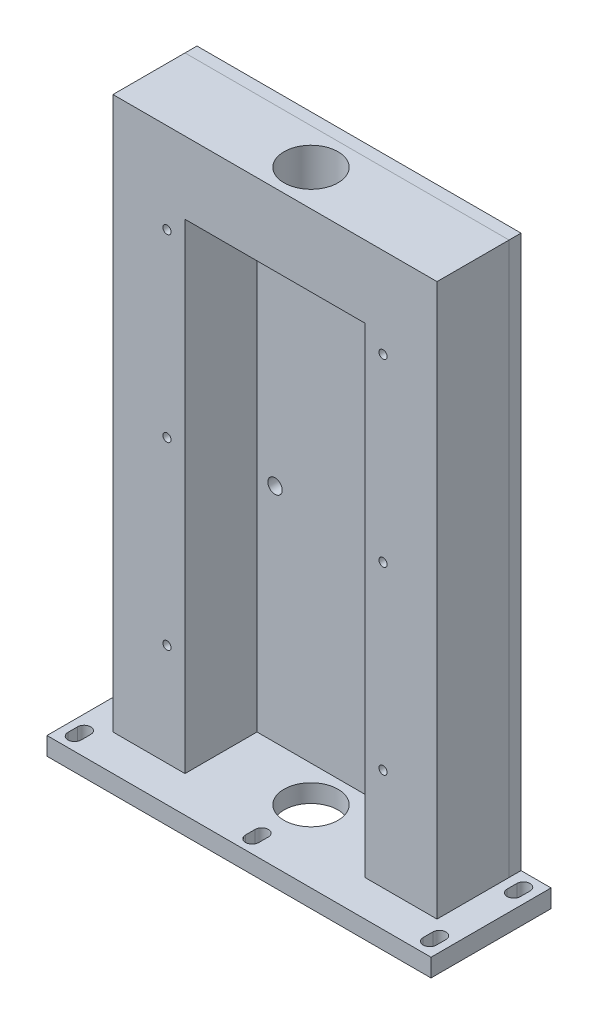
from build123d import *

# Parameters (mm, degrees)
BOSS_EXTRUDE1_DEPTH        = 60
SKETCH3_W                  = 270
SKETCH3_H                  = 460
BOSS_EXTRUDE3_DEPTH        = 10
SKETCH4_W                  = 320
SKETCH4_H                  = 100
BOSS_EXTRUDE4_DEPTH        = 15
SKETCH7_R                  = 5.5
CUT_EXTRUDE1_DEPTH         = 496.277699882
CUT_EXTRUDE3_DEPTH         = 496.277699882
SKETCH23_R                 = 22.5
CUT_EXTRUDE4_DEPTH         = 510.239629251
SKETCH24_R                 = 15
CUT_EXTRUDE5_DEPTH         = 498.192115786
SKETCH27_W                 = 3.4
SKETCH27_H                 = 100
M8_TAPPED_HOLE1_AT_2_COUNT = 2
M8_TAPPED_HOLE1_AT_2_PITCH = 180
M8_TAPPED_HOLE1_AT_3_COUNT = 2
M8_TAPPED_HOLE1_AT_3_PITCH = 150
M8_TAPPED_HOLE1_AT_4_COUNT = 2
M8_TAPPED_HOLE1_AT_4_PITCH = 234.307490277
M8_TAPPED_HOLE1_AT_5_COUNT = 2
M8_TAPPED_HOLE1_AT_5_PITCH = 300
M8_TAPPED_HOLE1_AT_6_COUNT = 2
M8_TAPPED_HOLE1_AT_6_PITCH = 349.857113691
SKETCH29_R                 = 6
CUT_EXTRUDE6_DEPTH         = 10


with BuildPart() as part:
    # Sketch1 → Boss-Extrude1 (new body)
    with BuildSketch(Plane.XY):
        Polygon((-135, 460), (135, 460), (135, 0), (75, 0), (75, 400), (-75, 400), (-75, 0), (-135, 0), align=None)
    extrude(amount=BOSS_EXTRUDE1_DEPTH)


with BuildPart() as body_2:
    # Sketch3 → Boss-Extrude3 (new body)
    with BuildSketch(Plane(origin=(0, 0, 0), x_dir=(-1, 0, 0), z_dir=(0, 0, -1))):
        with Locations((0, 230)):
            Rectangle(SKETCH3_W, SKETCH3_H)
    extrude(amount=BOSS_EXTRUDE3_DEPTH)

    # Sketch24 → Cut-Extrude5 (cut, through all)
    with BuildSketch(Plane(origin=(0, 0, -10), x_dir=(-1, 0, 0), z_dir=(0, 0, -1))):
        with Locations((-60, 257)):
            Circle(SKETCH24_R)
    extrude(amount=-CUT_EXTRUDE5_DEPTH, mode=Mode.SUBTRACT)


with BuildPart() as body_3:
    # Sketch4 → Boss-Extrude4 (new body)
    with BuildSketch(Plane.XZ):
        with Locations((0, 40)):
            Rectangle(SKETCH4_W, SKETCH4_H)
    extrude(amount=BOSS_EXTRUDE4_DEPTH)

    # Sketch7 → Cut-Extrude1 (cut, through all)
    with BuildSketch(Plane(origin=(0, 0, 0), x_dir=(1, 0, 0), z_dir=(0, 1, 0))):
        with Locations(Location((148, -5, 0), (0, 0, 270))):
            Circle(SKETCH7_R)
        with Locations(Location((148, -75, 0), (0, 0, 90))):
            Circle(SKETCH7_R)
        with Locations(Location((-148, -75, 0), (0, 0, 270))):
            Circle(SKETCH7_R)
        with Locations(Location((-148, -5, 0), (0, 0, 90))):
            Circle(SKETCH7_R)
        with Locations(Location((0, -75, 0), (0, 0, 270))):
            Circle(SKETCH7_R)
    extrude(amount=-CUT_EXTRUDE1_DEPTH, mode=Mode.SUBTRACT)

    # Sketch22 → Cut-Extrude3 (cut, through all)
    with BuildSketch(Plane(origin=(0, 0, 0), x_dir=(1, 0, 0), z_dir=(0, 1, 0))):
        with BuildLine():
            Line((-142.5, -1), (-142.5, -9))
            ThreePointArc((-142.5, -9), (-148, -14.5), (-153.5, -9))
            Line((-153.5, -9), (-153.5, -1))
            ThreePointArc((-153.5, -1), (-148, 4.5), (-142.5, -1))
        make_face()
        with BuildLine():
            Line((-142.5, -71), (-142.5, -79))
            ThreePointArc((-142.5, -79), (-148, -84.5), (-153.5, -79))
            Line((-153.5, -79), (-153.5, -71))
            ThreePointArc((-153.5, -71), (-148, -65.5), (-142.5, -71))
        make_face()
        with BuildLine():
            Line((142.5, -1), (142.5, -9))
            ThreePointArc((142.5, -9), (148, -14.5), (153.5, -9))
            Line((153.5, -9), (153.5, -1))
            ThreePointArc((153.5, -1), (148, 4.5), (142.5, -1))
        make_face()
        with BuildLine():
            Line((142.5, -71), (142.5, -79))
            ThreePointArc((142.5, -79), (148, -84.5), (153.5, -79))
            Line((153.5, -79), (153.5, -71))
            ThreePointArc((153.5, -71), (148, -65.5), (142.5, -71))
        make_face()
        with BuildLine():
            Line((5.5, -71), (5.5, -79))
            ThreePointArc((5.5, -79), (0, -84.5), (-5.5, -79))
            Line((-5.5, -79), (-5.5, -71))
            ThreePointArc((-5.5, -71), (0, -65.5), (5.5, -71))
        make_face()
    extrude(amount=-CUT_EXTRUDE3_DEPTH, mode=Mode.SUBTRACT)


with BuildPart() as cut_extrude4_tool:
    # Sketch23 → Cut-Extrude4 (new, through all)
    with BuildSketch(Plane(origin=(0, 460, 0), x_dir=(1, 0, 0), z_dir=(0, 1, 0))):
        with Locations(Location((0, -30, 0), (0, 0, 270))):
            Circle(SKETCH23_R)
    extrude(amount=-CUT_EXTRUDE4_DEPTH)


with BuildPart() as part_1:
    add(part.part)

    # Cut-Extrude4: cut by cut_extrude4_tool
    add(cut_extrude4_tool.part, mode=Mode.SUBTRACT)


with BuildPart() as body_3_1:
    add(body_3.part)

    # Cut-Extrude4: cut by cut_extrude4_tool
    add(cut_extrude4_tool.part, mode=Mode.SUBTRACT)


with BuildPart() as m8_tapped_hole1_tool:
    # Sketch27 → M8 Tapped Hole1 (revolve)
    with BuildSketch(Plane(origin=(90, 385, -10), x_dir=(0, 1, 0), z_dir=(1, 0, 0))):
        with Locations((1.7, 50)):
            Rectangle(SKETCH27_W, SKETCH27_H)
    m8_tapped_hole1 = revolve(axis=Axis((90, 385, -16.35), (0, 0, 1)))


with BuildPart() as part_2:
    add(part_1.part)

    # M8 Tapped Hole1: cut by m8_tapped_hole1_tool
    add(m8_tapped_hole1_tool.part, mode=Mode.SUBTRACT)


with BuildPart() as body_2_1:
    add(body_2.part)

    # M8 Tapped Hole1: cut by m8_tapped_hole1_tool
    add(m8_tapped_hole1_tool.part, mode=Mode.SUBTRACT)


with BuildPart() as m8_tapped_hole1_at_2_tool:
    # M8 Tapped Hole1 at 2: M8 Tapped Hole1 ×2
    with Locations(*[(-i * M8_TAPPED_HOLE1_AT_2_PITCH, 0, 0) for i in range(1, M8_TAPPED_HOLE1_AT_2_COUNT)]):
        add(m8_tapped_hole1)


with BuildPart() as part_3:
    add(part_2.part)

    # M8 Tapped Hole1 at 2: cut by m8_tapped_hole1_at_2_tool
    add(m8_tapped_hole1_at_2_tool.part, mode=Mode.SUBTRACT)


with BuildPart() as body_2_2:
    add(body_2_1.part)

    # M8 Tapped Hole1 at 2: cut by m8_tapped_hole1_at_2_tool
    add(m8_tapped_hole1_at_2_tool.part, mode=Mode.SUBTRACT)


with BuildPart() as m8_tapped_hole1_at_3_tool:
    # M8 Tapped Hole1 at 3: M8 Tapped Hole1 ×2
    with Locations(*[(0, -i * M8_TAPPED_HOLE1_AT_3_PITCH, 0) for i in range(1, M8_TAPPED_HOLE1_AT_3_COUNT)]):
        add(m8_tapped_hole1)


with BuildPart() as part_4:
    add(part_3.part)

    # M8 Tapped Hole1 at 3: cut by m8_tapped_hole1_at_3_tool
    add(m8_tapped_hole1_at_3_tool.part, mode=Mode.SUBTRACT)


with BuildPart() as body_2_3:
    add(body_2_2.part)

    # M8 Tapped Hole1 at 3: cut by m8_tapped_hole1_at_3_tool
    add(m8_tapped_hole1_at_3_tool.part, mode=Mode.SUBTRACT)


with BuildPart() as m8_tapped_hole1_at_4_tool:
    # M8 Tapped Hole1 at 4: M8 Tapped Hole1 ×2
    with Locations(*[Vector(-0.7682212795973759, -0.6401843996644798, 0) * (i * M8_TAPPED_HOLE1_AT_4_PITCH) for i in range(1, M8_TAPPED_HOLE1_AT_4_COUNT)]):
        add(m8_tapped_hole1)


with BuildPart() as part_5:
    add(part_4.part)

    # M8 Tapped Hole1 at 4: cut by m8_tapped_hole1_at_4_tool
    add(m8_tapped_hole1_at_4_tool.part, mode=Mode.SUBTRACT)


with BuildPart() as body_2_4:
    add(body_2_3.part)

    # M8 Tapped Hole1 at 4: cut by m8_tapped_hole1_at_4_tool
    add(m8_tapped_hole1_at_4_tool.part, mode=Mode.SUBTRACT)


with BuildPart() as m8_tapped_hole1_at_5_tool:
    # M8 Tapped Hole1 at 5: M8 Tapped Hole1 ×2
    with Locations(*[(0, -i * M8_TAPPED_HOLE1_AT_5_PITCH, 0) for i in range(1, M8_TAPPED_HOLE1_AT_5_COUNT)]):
        add(m8_tapped_hole1)


with BuildPart() as part_6:
    add(part_5.part)

    # M8 Tapped Hole1 at 5: cut by m8_tapped_hole1_at_5_tool
    add(m8_tapped_hole1_at_5_tool.part, mode=Mode.SUBTRACT)


with BuildPart() as body_2_5:
    add(body_2_4.part)

    # M8 Tapped Hole1 at 5: cut by m8_tapped_hole1_at_5_tool
    add(m8_tapped_hole1_at_5_tool.part, mode=Mode.SUBTRACT)


with BuildPart() as m8_tapped_hole1_at_6_tool:
    # M8 Tapped Hole1 at 6: M8 Tapped Hole1 ×2
    with Locations(*[Vector(-0.5144957554275266, -0.8574929257125442, 0) * (i * M8_TAPPED_HOLE1_AT_6_PITCH) for i in range(1, M8_TAPPED_HOLE1_AT_6_COUNT)]):
        add(m8_tapped_hole1)


with BuildPart() as part_7:
    add(part_6.part)

    # M8 Tapped Hole1 at 6: cut by m8_tapped_hole1_at_6_tool
    add(m8_tapped_hole1_at_6_tool.part, mode=Mode.SUBTRACT)


with BuildPart() as body_2_6:
    add(body_2_5.part)

    # M8 Tapped Hole1 at 6: cut by m8_tapped_hole1_at_6_tool
    add(m8_tapped_hole1_at_6_tool.part, mode=Mode.SUBTRACT)

    # Sketch29 → Cut-Extrude6 (cut)
    with BuildSketch(Plane(origin=(0, 0, -10), x_dir=(-1, 0, 0), z_dir=(0, 0, -1))):
        with Locations((-60, 185)):
            Circle(SKETCH29_R)
        with Locations(Location((60, 185, 0), (0, 0, 180))):
            Circle(SKETCH29_R)
    extrude(amount=-CUT_EXTRUDE6_DEPTH, mode=Mode.SUBTRACT)


solid = Compound([body_3_1.part, part_7.part, body_2_6.part])
